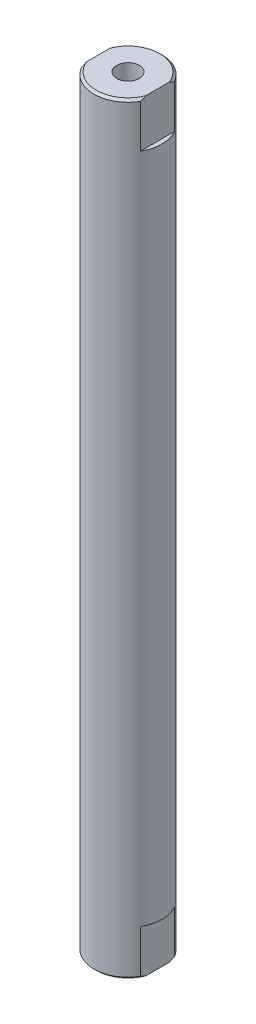
SolidWorks part; units mm, degrees
material "A6061"
ref_plane "前基準面" through (0, 0, 0) normal (0, 0, 1) x (1, 0, 0)
ref_plane "上基準面" through (0, 0, 0) normal (0, 1, 0) x (1, 0, 0)
ref_plane "右基準面" through (0, 0, 0) normal (1, 0, 0) x (0, 0, -1)
sketch "草图1" plane through (0, 0, 0) normal (0, 1, 0) x (1, 0, 0)
  circle A0 centre (0, 0) radius 7.5
  dimension "D1" = 15
extrude "凸台-拉伸1" add sketch "草图1" along normal mid plane 168
chamfer "倒角1" distance 0.5 angle 45 2 edges at (0, -84, 7.5) (0, 84, 7.5)
hole_wizard "M6 螺纹孔1" positions "草图3" profile "草图2" tap size "M6" standard "GB"
sketch "草图3" plane through (0, 84, 0) normal (0, 1, 0) x (1, 0, 0)
  point P0 (0, 0)
sketch "草图2" plane through (0, 84, 0) normal (1, 0, 0) x (0, 0, 1)
  line L0 (0, 0) -> (0, 18.5022)
  line L1 (0, 18.5022) -> (2.5, 17)
  line L2 (2.5, 17) -> (2.5, 0)
  line L5 (2.5, 0) -> (0, 0)
  line L10 (0, 18.5022) -> (-2.5, 17) construction
  line L11 (0, -6.35) -> (0, 107.95) construction
  dimension "螺纹孔钻头直径" = 5
  dimension "螺纹孔钻头深度" = 17
  dimension "导头角度" = 118
cosmetic thread "孔螺蚊线1" parameters "D1"=12, "D2"=6
mirror "镜向1" about plane through (0, 0, 0) normal (0, 1, 0) of "M6 螺纹孔1"
sketch "草图4" plane through (0, 0, 0) normal (0, 0, 1) x (1, 0, 0)
  line L0 (-7.5, 83.5) -> (-7.5, -83.5) construction
  line L1 (-7.5, 74) -> (-6.5, 74)
  line L2 (-7.5, 74) -> (-7.5, 84)
  line L3 (-7.5, 84) -> (-6.5, 84)
  line L4 (-6.5, 74) -> (-6.5, 84)
  line L5 (7, 84) -> (-7, 84) construction
  line L6 (0, 82.6256) -> (0, 0) construction
  line L7 (0, 0) -> (-19.2395, 0) construction
  line L8 (6.5, 74) -> (6.5, 84)
  line L9 (7.5, 84) -> (6.5, 84)
  line L10 (7.5, 74) -> (7.5, 84)
  line L11 (7.5, 74) -> (6.5, 74)
  line L12 (7.5, -74) -> (6.5, -74)
  line L13 (7.5, -74) -> (7.5, -84)
  line L14 (7.5, -84) -> (6.5, -84)
  line L15 (6.5, -74) -> (6.5, -84)
  line L16 (-6.5, -74) -> (-6.5, -84)
  line L17 (-7.5, -84) -> (-6.5, -84)
  line L18 (-7.5, -74) -> (-7.5, -84)
  line L19 (-7.5, -74) -> (-6.5, -74)
  dimension "D1" = 1
  dimension "D2" = 10
extrude "切除-拉伸1" cut sketch "草图4" against normal mid plane 20
